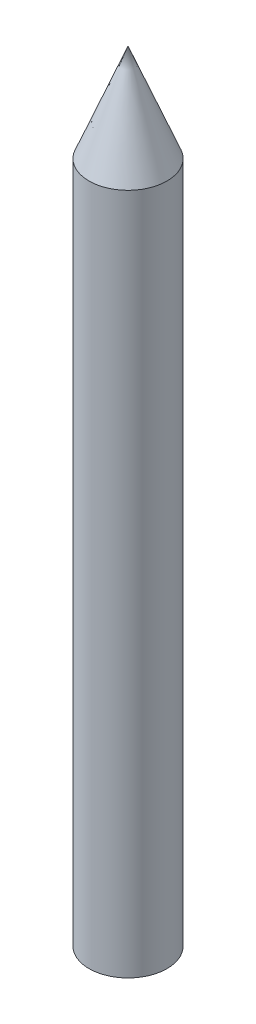
from build123d import *


with BuildPart() as part:
    # 草图1 → 旋转1 (revolve)
    with BuildSketch(Plane.XY, mode=Mode.PRIVATE) as revolve_1_sk:
        Polygon((0, 0), (0, 80), (-4, 70), (-4, 0), align=None)
    revolve(revolve_1_sk.sketch.rotate(Axis((0, 0, 0), (0, 1, 0)), 270), axis=Axis((0, 0, 0), (0, 1, 0)))


solid = part.part
